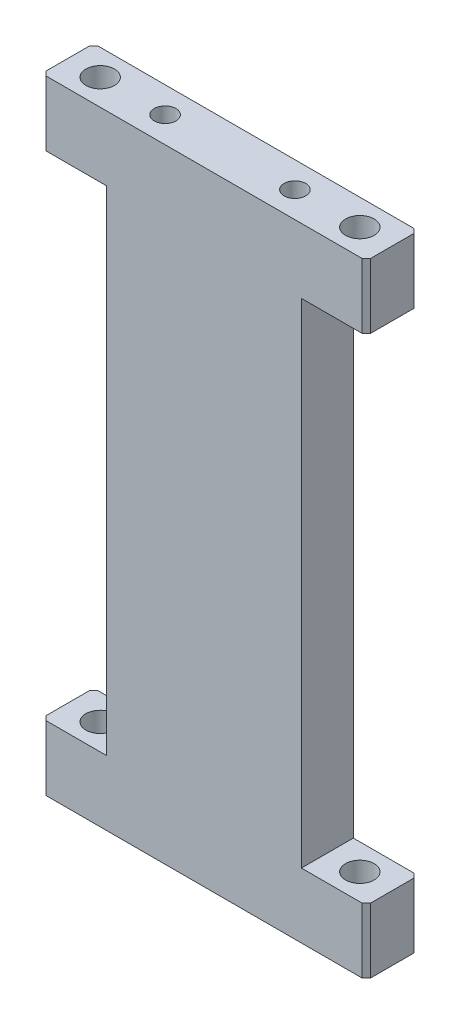
from build123d import *

# Parameters (mm, degrees)
SKETCH1_W                          = 75
SKETCH1_H                          = 144
BOSS_EXTRUDE1_DEPTH                = 6
SKETCH4_W                          = 15
SKETCH4_H                          = 114
CUT_EXTRUDE1_DEPTH                 = 83.0624762
F_6_6_6_6_DIAMETER_HOLE1_D         = 6.6
BLIND_PIN_HOLE1_SIZE_MM_AT_2_COUNT = 2
BLIND_PIN_HOLE1_SIZE_MM_AT_2_PITCH = 30
CHAMFER1_SIZE                      = 1


with BuildPart() as part:
    # Sketch1 → Boss-Extrude1 (new, symmetric)
    with BuildSketch(Plane.XY):
        Rectangle(SKETCH1_W, SKETCH1_H)
    extrude(amount=BOSS_EXTRUDE1_DEPTH, both=True)

    # Sketch4 → Cut-Extrude1 (cut, through all)
    with BuildSketch(Plane.XY.offset(6)):
        with Locations((-30, 0)):
            Rectangle(SKETCH4_W, SKETCH4_H)
    cut_extrude1 = extrude(amount=-CUT_EXTRUDE1_DEPTH, mode=Mode.SUBTRACT)

    # Mirror1: Cut-Extrude1 across plane
    add(cut_extrude1.mirror(Plane(origin=(0, 0, 0), x_dir=(0, 0, 1), z_dir=(1, 0, 0))), mode=Mode.SUBTRACT)

    # Ø6.6 (6.6) Diameter Hole1 (through all)
    with Locations(Plane(origin=(0, -72, 0), x_dir=(-1, 0, 0), z_dir=(0, -1, 0))):
        with Locations((-30, 0), (30, 0)):
            Hole(F_6_6_6_6_DIAMETER_HOLE1_D / 2)

    # Sketch8 → Blind Pin Hole1 (size mm) (revolve, cut)
    with BuildSketch(Plane(origin=(15, -72, 0), x_dir=(0, 0, -1), z_dir=(1, 0, 0))):
        Polygon((0, 0), (0, 12.502151548), (2.5, 11), (2.5, 0), align=None)
    blind_pin_hole1_size_mm = revolve(axis=Axis((15, -78.35, 0), (0, 1, 0)), mode=Mode.SUBTRACT)

    # Blind Pin Hole1 (size mm) at 2: Blind Pin Hole1 (size mm) ×2
    with Locations(*[(-i * BLIND_PIN_HOLE1_SIZE_MM_AT_2_PITCH, 0, 0) for i in range(1, BLIND_PIN_HOLE1_SIZE_MM_AT_2_COUNT)]):
        add(blind_pin_hole1_size_mm, mode=Mode.SUBTRACT)

    # Mirror2: Blind Pin Hole1 (size mm) across plane
    add(blind_pin_hole1_size_mm.mirror(Plane.ZX), mode=Mode.SUBTRACT)

    # Mirror2 copy 1 sketch → Mirror2 copy 1 (revolve, cut)
    with BuildSketch(Plane(origin=(-15, 72, 0), x_dir=(0, 0, -1), z_dir=(1, 0, 0))):
        Polygon((0, 0), (0, -12.502151548), (2.5, -11), (2.5, 0), align=None)
    revolve(axis=Axis((-15, 78.35, 0), (0, 1, 0)), mode=Mode.SUBTRACT)

    # Chamfer1
    chamfer1_edges = [part.edges().sort_by_distance(p)[0] for p in [
        (-37.5, 64.5, 6),
        (-37.5, -64.5, -6),
        (-37.5, -64.5, 6),
        (37.5, 64.5, -6),
        (37.5, 64.5, 6),
        (37.5, -64.5, 6),
        (-37.5, 64.5, -6),
        (37.5, -64.5, -6),
    ]]
    chamfer(chamfer1_edges, length=CHAMFER1_SIZE)


solid = part.part
